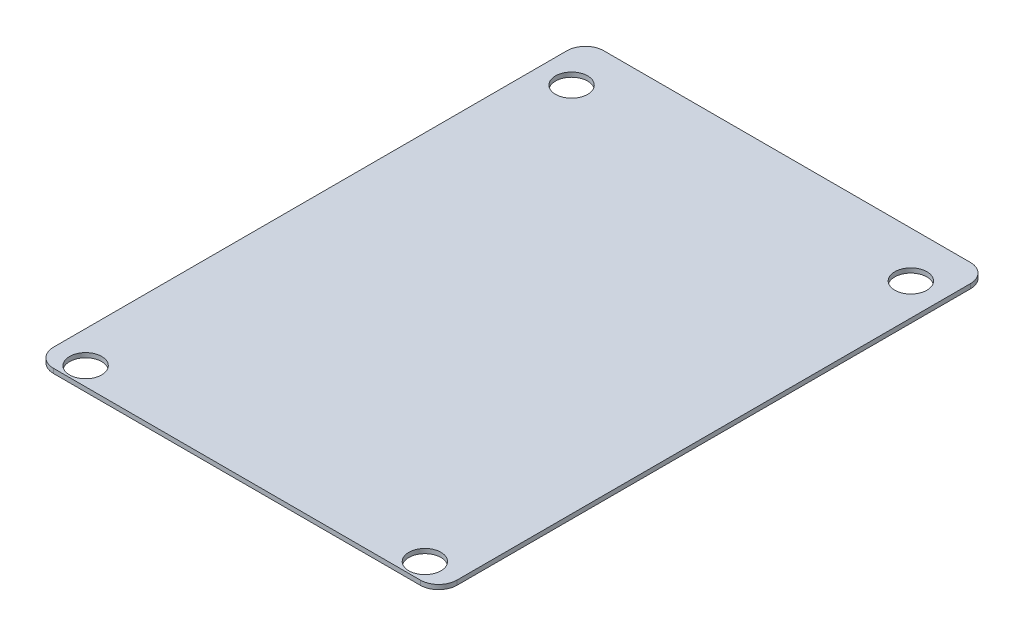
SolidWorks part; units mm, degrees
material "橡胶"
ref_plane "Front Plane" through (0, 0, 0) normal (0, 0, 1) x (1, 0, 0)
ref_plane "Top Plane" through (0, 0, 0) normal (0, 1, 0) x (1, 0, 0)
ref_plane "Right Plane" through (0, 0, 0) normal (1, 0, 0) x (0, 0, -1)
sketch "Sketch1" plane through (0, 0, 0) normal (0, 1, 0) x (1, 0, 0)
  line L1 (-69.85, 100.0125) -> (69.85, 100.0125)
  line L2 (-69.85, 100.0125) -> (-69.85, -90.4875)
  line L3 (-69.85, -90.4875) -> (69.85, -90.4875)
  line L4 (69.85, 100.0125) -> (69.85, -90.4875)
  dimension "D1" = 100.0125
  dimension "D2" = 190.5
  dimension "D3" = 69.85
  dimension "D4" = 139.7
extrude "Boss-Extrude1" add sketch "Sketch1" along normal blind 1.5748
fillet "Fillet1" radius 6.35 4 edges at (-69.85, 0.7874, -100.0125) (69.85, 0.7874, -100.0125) (69.85, 0.7874, 90.4875) (-69.85, 0.7874, 90.4875)
hole_wizard "7/16 (0.4375) Diameter Hole1" positions "Sketch3" profile "Sketch2" hole size "7/16" standard "Ansi Inch" end condition through all
sketch "Sketch3" plane through (0, 1.5748, 0) normal (0, 1, 0) x (1, 0, 0)
  line L0 (63.5, 100.0125) -> (-63.5, 100.0125) construction
  line L2 (-69.85, 93.6625) -> (-69.85, -84.1375) construction
  point P0 (-58.738, 84.1375)
  dimension "D1" = 15.875
  dimension "D2" = 11.112
sketch "Sketch2" plane through (-58.738, 1.5748, -84.1375) normal (1, 0, 0) x (0, 0, 1)
  line L0 (0, 0) -> (0, 1.5748)
  line L1 (0, 1.5748) -> (5.5562, 1.5748)
  line L2 (5.5562, 1.5748) -> (5.5562, 0)
  line L5 (5.5562, 0) -> (0, 0)
  line L11 (0, -6.35) -> (0, 107.95) construction
  dimension "通孔孔直径" = 11.1125
  dimension "通孔孔深度" = 1.5748
pattern_linear "LPattern1" count 2 spacing 168.275 along (0, 0, 1) count 2 spacing 117.475 along (1, 0, 0) of "7/16 (0.4375) Diameter Hole1"
